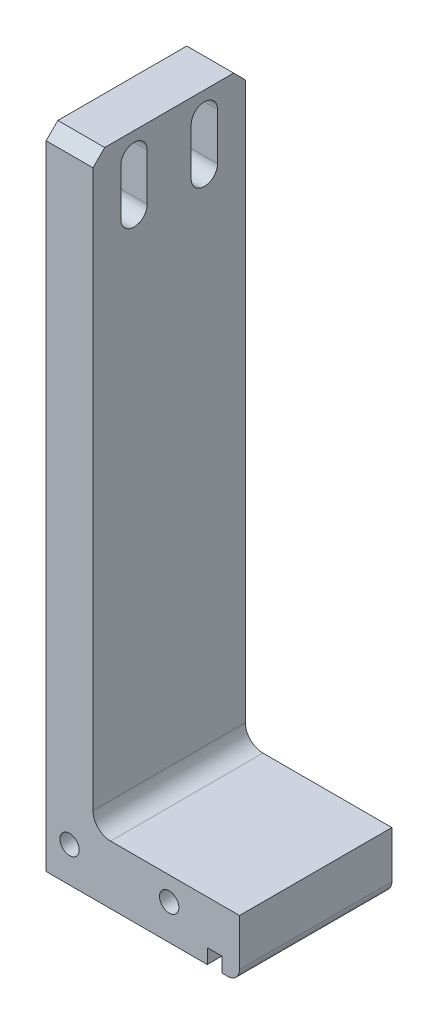
from build123d import *

# Parameters (mm, degrees)
BOSS_EXTRUDE1_DEPTH   = 13
SKETCH2_W             = 2.5
SKETCH2_H             = 2.5
CUT_EXTRUDE1_DEPTH    = 118.749734607
M4_TAPPED_HOLE1_D     = 3.3
M4_TAPPED_HOLE1_DEPTH = 10.1
M3_TAPPED_HOLE1_D     = 2.5
M3_TAPPED_HOLE1_DEPTH = 7.5
CUT_EXTRUDE2_DEPTH    = 114.551750317
FILLET1_R             = 2
FILLET2_R             = 3
CHAMFER1_SIZE         = 2


with BuildPart() as part:
    # Sketch1 → Boss-Extrude1 (new, symmetric)
    with BuildSketch(Plane.XY):
        Polygon((0, 110), (8, 110), (8, 10), (33, 10), (33, 0), (0, 0), align=None)
    extrude(amount=BOSS_EXTRUDE1_DEPTH, both=True)

    # Sketch2 → Cut-Extrude1 (cut, through all)
    with BuildSketch(Plane.XY.offset(13)):
        with Locations((28.75, 1.25)):
            Rectangle(SKETCH2_W, SKETCH2_H)
    extrude(amount=-CUT_EXTRUDE1_DEPTH, mode=Mode.SUBTRACT)

    # M4 Tapped Hole1
    with Locations(Plane.XY.offset(13)):
        with Locations((21, 6), (4, 6)):
            m4_tapped_hole1 = Hole(M4_TAPPED_HOLE1_D / 2, depth=M4_TAPPED_HOLE1_DEPTH)

    # Mirror1: M4 Tapped Hole1 across plane
    add(m4_tapped_hole1.mirror(Plane.XY), mode=Mode.SUBTRACT)

    # M3 Tapped Hole1
    with Locations(Plane.XZ):
        with Locations((25, 8), (9, 8), (9, -8), (25, -8)):
            Hole(M3_TAPPED_HOLE1_D / 2, depth=M3_TAPPED_HOLE1_DEPTH)

    # Sketch7 → Cut-Extrude2 (cut, through all)
    with BuildSketch(Plane(origin=(8, 0, 0), x_dir=(0, 0, -1), z_dir=(1, 0, 0))):
        with BuildLine():
            Line((-3.75, 106), (-3.75, 98))
            ThreePointArc((-3.75, 98), (-6, 95.75), (-8.25, 98))
            Line((-8.25, 98), (-8.25, 106))
            ThreePointArc((-8.25, 106), (-6, 108.25), (-3.75, 106))
        make_face()
        with BuildLine():
            Line((3.75, 106), (3.75, 98))
            ThreePointArc((3.75, 98), (6, 95.75), (8.25, 98))
            Line((8.25, 98), (8.25, 106))
            ThreePointArc((8.25, 106), (6, 108.25), (3.75, 106))
        make_face()
    extrude(amount=-CUT_EXTRUDE2_DEPTH, mode=Mode.SUBTRACT)

    # Fillet1
    fillet1_edges = [part.edges().sort_by_distance(p)[0] for p in [
        (33, 0, 0),
    ]]
    fillet(fillet1_edges, radius=FILLET1_R)

    # Fillet2
    fillet2_edges = [part.edges().sort_by_distance(p)[0] for p in [
        (8, 10, 0),
    ]]
    fillet(fillet2_edges, radius=FILLET2_R)

    # Chamfer1
    chamfer1_edges = [part.edges().sort_by_distance(p)[0] for p in [
        (4, 110, 13),
        (4, 110, -13),
    ]]
    chamfer(chamfer1_edges, length=CHAMFER1_SIZE)


solid = part.part
